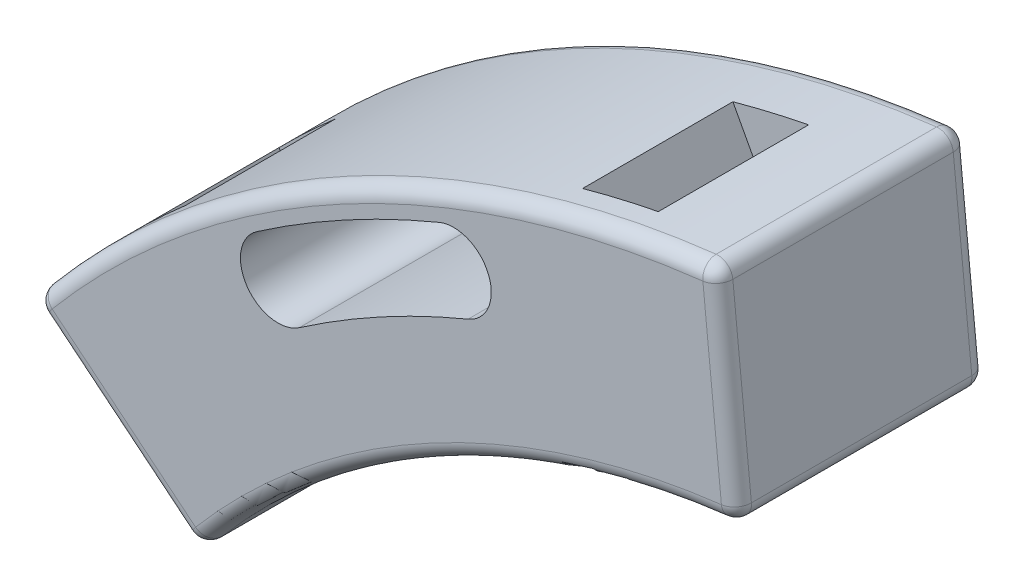
SolidWorks part; units mm, degrees
ref_plane "Front Plane" through (0, 0, 0) normal (0, 0, 1) x (1, 0, 0)
ref_plane "Top Plane" through (0, 0, 0) normal (0, 1, 0) x (1, 0, 0)
ref_plane "Right Plane" through (0, 0, 0) normal (1, 0, 0) x (0, 0, -1)
other "Configuration Table"
sketch "Sketch1" plane through (0, 0, 0) normal (0, 0, 1) x (1, 0, 0)
  line L0 (-307.586, 341.8878) -> (-311.8851, 384.6509)
  line L1 (-415.4405, 283.9575) -> (-448.7186, 311.1557)
  arc A0 (-307.586, 341.8878) -> (-415.4405, 283.9575) centre (-291.5852, 182.7307) ccw
  arc A1 (-311.8851, 384.6509) -> (-448.7186, 311.1557) centre (-291.5852, 182.7307) ccw
  arc A2 (-309.7355, 363.2694) -> (-432.0795, 297.5566) centre (-291.5852, 182.7307) ccw construction
  arc A3 (-265.8435, 428.1061) -> (-262.6089, 355.5583) centre (-280.9901, 391.0848) ccw construction
  circle A4 centre (-341.3111, 367.4404) radius 7.5 construction
  dimension "D1" = 45
  dimension "D2" = 31
extrude "Boss-Extrude1" add sketch "Sketch1" along normal blind 50
ref_plane "Plane1" through (-150.1273, -80.6356, 0) normal (-0.881, -0.4732, 0) x (0, 0, 1)
ref_plane "Plane2" through (-237.4841, 442.1478, 0) normal (-0.4732, 0.881, 0) x (0.881, 0.4732, 0)
sketch "Sketch2" plane through (-237.4841, 442.1478, 0) normal (-0.4732, 0.881, 0) x (0.881, 0.4732, 0)
  line L0 (-215.4122, -28) -> (-125.4122, -28) construction
  line L1 (-215.4122, -43) -> (-230.4122, -43)
  line L2 (-215.4122, -43) -> (-215.4122, -13)
  line L3 (-215.4122, -13) -> (-230.4122, -13)
  line L4 (-230.4122, -43) -> (-230.4122, -13)
  line L5 (-215.4122, -43) -> (-230.4122, -13) construction
  line L6 (-215.4122, -13) -> (-230.4122, -43) construction
  line L7 (-110.4122, -43) -> (-125.4122, -43)
  line L8 (-110.4122, -43) -> (-110.4122, -13)
  line L9 (-110.4122, -13) -> (-125.4122, -13)
  line L10 (-125.4122, -43) -> (-125.4122, -13)
  line L11 (-110.4122, -43) -> (-125.4122, -13) construction
  line L12 (-110.4122, -13) -> (-125.4122, -43) construction
  line L13 (-92.7511, 0) -> (-248.0732, 0) construction
  line L14 (-170.4122, -28) -> (-170.4122, 0) construction
  point P0 (-222.9122, -28)
  point P5 (-117.9122, -28)
  dimension "D1" = 15
  dimension "D2" = 30
  dimension "D3" = 28
  dimension "D4" = 90
extrude "Cut-Extrude1" cut sketch "Sketch2" against normal blind 20
sketch "Sketch3" plane through (0, 0, 0) normal (0, 0, -1) x (-1, 0, 0)
  arc A0 (364.3142, 358.2599) -> (399.3896, 339.1859) centre (291.5852, 182.7307) cw construction
  arc A5 (403.645, 345.3617) -> (367.1851, 365.1887) centre (291.5852, 182.7307) ccw
  arc A6 (395.1341, 333.01) -> (361.4433, 351.3311) centre (291.5852, 182.7307) ccw
  arc A7 (395.1341, 333.01) -> (403.645, 345.3617) centre (399.3896, 339.1859) ccw
  arc A8 (367.1851, 365.1887) -> (361.4433, 351.3311) centre (364.3142, 358.2599) ccw
  point P3 (382.3543, 349.6468)
  dimension "D1" = 190
  dimension "D2" = 7.5
extrude "Cut-Extrude2" cut sketch "Sketch3" against normal through all both and the other way through all
fillet "Fillet1" radius 3 12 edges at (-367.2748, 323.6495, 0) (-309.7355, 363.2694, 0) (-387.6114, 361.5122, 0) (-432.0795, 297.5566, 0) (-367.2748, 323.6495, 50) (-309.7355, 363.2694, 50) (-387.6114, 361.5122, 50) (-415.4405, 283.9575, 25) (-448.7186, 311.1557, 25) (-311.8851, 384.6509, 25) (-307.586, 341.8878, 25) (-432.0795, 297.5566, 50)
